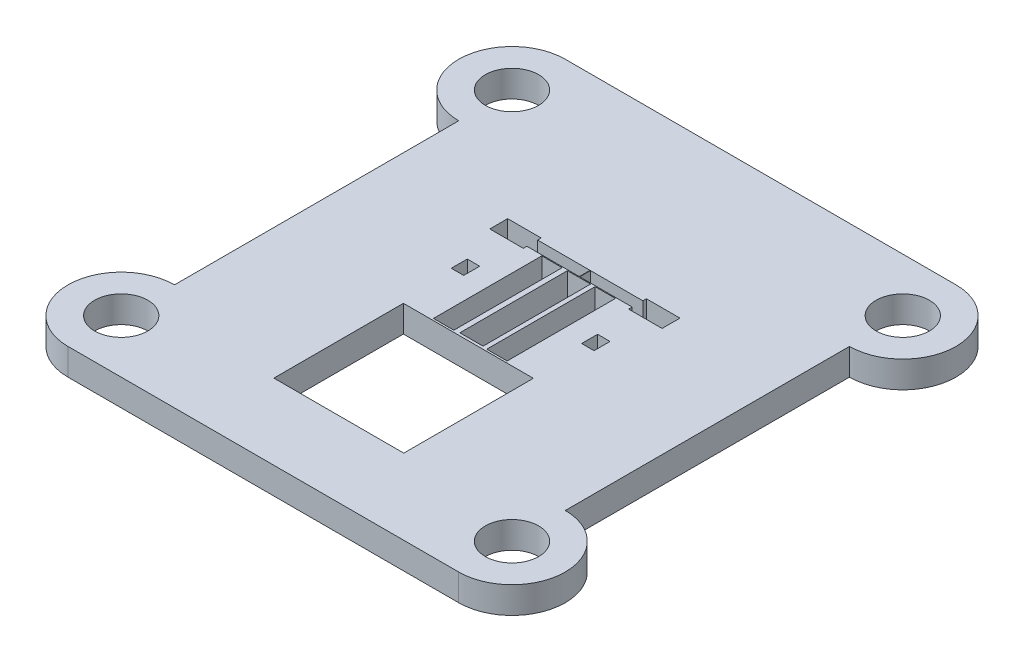
from build123d import *

# Parameters (mm, degrees)
SKETCH1_R           = 15
BOSS_EXTRUDE1_DEPTH = 15
CUT_EXTRUDE1_REACH  = 200.557
SKETCH6_W           = 73.144376366
SKETCH6_H           = 72.943161699
SKETCH6_W_2         = 11.5
SKETCH6_H_2         = 61
SKETCH6_W_3         = 13.06
SKETCH6_H_3         = 60.56
SKETCH6_W_4         = 7
SKETCH6_H_4         = 9
SKETCH7_W           = 22
SKETCH7_H           = 52
CUT_EXTRUDE2_DEPTH  = 10
FILLET1_R           = 1


with BuildPart() as part:
    # Sketch1 → Boss-Extrude1 (new body)
    with BuildSketch(Plane(origin=(0, 0, 0), x_dir=(1, 0, 0), z_dir=(0, 1, 0))):
        with BuildLine():
            Line((-110, -140), (80, -140))
            Line((80, -140), (80, 140))
            Line((80, 140), (-110, 140))
            ThreePointArc((-110, 140), (-140, 110), (-110, 80))
            Line((-110, 80), (-110, -80))
            ThreePointArc((-110, -80), (-140, -110), (-110, -140))
        make_face()
        with Locations(Location((-110, 110, 0), (0, 0, 270))):
            Circle(SKETCH1_R, mode=Mode.SUBTRACT)
        with Locations(Location((-110, -110, 0), (0, 0, 270))):
            Circle(SKETCH1_R, mode=Mode.SUBTRACT)
    boss_extrude1 = extrude(amount=BOSS_EXTRUDE1_DEPTH)

    # Mirror1: Boss-Extrude1 across plane
    add(boss_extrude1.mirror(Plane(origin=(0, 0, 0), x_dir=(0, 0, 1), z_dir=(1, 0, 0))))

    # Sketch6 → Cut-Extrude1 (cut, up to next)
    with BuildSketch(Plane(origin=(0, 15, 0), x_dir=(1, 0, 0), z_dir=(0, 1, 0)), mode=Mode.PRIVATE) as cut_extrude1_sk1:
        with Locations((0, -61.02841915)):
            Rectangle(SKETCH6_W, SKETCH6_H)
    cut_extrude1_tool1 = extrude(cut_extrude1_sk1.sketch, amount=-CUT_EXTRUDE1_REACH, mode=Mode.PRIVATE) & part.part
    # Sketch6 → Cut-Extrude1 (cut, up to next)
    with BuildSketch(Plane(origin=(0, 15, 0), x_dir=(1, 0, 0), z_dir=(0, 1, 0)), mode=Mode.PRIVATE) as cut_extrude1_sk2:
        with Locations((-15, 7)):
            Rectangle(SKETCH6_W_2, SKETCH6_H_2)
    cut_extrude1_tool2 = extrude(cut_extrude1_sk2.sketch, amount=-CUT_EXTRUDE1_REACH, mode=Mode.PRIVATE) & part.part
    # Sketch6 → Cut-Extrude1 (cut, up to next)
    with BuildSketch(Plane(origin=(0, 15, 0), x_dir=(1, 0, 0), z_dir=(0, 1, 0)), mode=Mode.PRIVATE) as cut_extrude1_sk3:
        Polygon((-0.14, 38), (-0.14, 44.06), (-29.63, 44.06), (-29.63, 46.06), (-48.5, 46.06), (-48.5, 36), (-29.63, 36), (-29.63, 38), align=None)
    cut_extrude1_tool3 = extrude(cut_extrude1_sk3.sketch, amount=-CUT_EXTRUDE1_REACH, mode=Mode.PRIVATE) & part.part
    # Sketch6 → Cut-Extrude1 (cut, up to next)
    with BuildSketch(Plane(origin=(0, 15, 0), x_dir=(1, 0, 0), z_dir=(0, 1, 0)), mode=Mode.PRIVATE) as cut_extrude1_sk4:
        Polygon((29.63, 36), (48.5, 36), (48.5, 46.06), (29.63, 46.06), (29.63, 44.06), (0.14, 44.06), (0.14, 38), (29.63, 38), align=None)
    cut_extrude1_tool4 = extrude(cut_extrude1_sk4.sketch, amount=-CUT_EXTRUDE1_REACH, mode=Mode.PRIVATE) & part.part
    # Sketch6 → Cut-Extrude1 (cut, up to next)
    with BuildSketch(Plane(origin=(0, 15, 0), x_dir=(1, 0, 0), z_dir=(0, 1, 0)), mode=Mode.PRIVATE) as cut_extrude1_sk5:
        with Locations((0.22, 7.22)):
            Rectangle(SKETCH6_W_3, SKETCH6_H_3)
    cut_extrude1_tool5 = extrude(cut_extrude1_sk5.sketch, amount=-CUT_EXTRUDE1_REACH, mode=Mode.PRIVATE) & part.part
    # Sketch6 → Cut-Extrude1 (cut, up to next)
    with BuildSketch(Plane(origin=(0, 15, 0), x_dir=(1, 0, 0), z_dir=(0, 1, 0)), mode=Mode.PRIVATE) as cut_extrude1_sk6:
        with Locations((15, 7)):
            Rectangle(SKETCH6_W_2, SKETCH6_H_2)
    cut_extrude1_tool6 = extrude(cut_extrude1_sk6.sketch, amount=-CUT_EXTRUDE1_REACH, mode=Mode.PRIVATE) & part.part
    # Sketch6 → Cut-Extrude1 (cut, up to next)
    with BuildSketch(Plane(origin=(0, 15, 0), x_dir=(1, 0, 0), z_dir=(0, 1, 0)), mode=Mode.PRIVATE) as cut_extrude1_sk7:
        with Locations((-36.69, 10.5)):
            Rectangle(SKETCH6_W_4, SKETCH6_H_4)
    cut_extrude1_tool7 = extrude(cut_extrude1_sk7.sketch, amount=-CUT_EXTRUDE1_REACH, mode=Mode.PRIVATE) & part.part
    # Sketch6 → Cut-Extrude1 (cut, up to next)
    with BuildSketch(Plane(origin=(0, 15, 0), x_dir=(1, 0, 0), z_dir=(0, 1, 0)), mode=Mode.PRIVATE) as cut_extrude1_sk8:
        with Locations((36.69, 10.5)):
            Rectangle(SKETCH6_W_4, SKETCH6_H_4)
    cut_extrude1_tool8 = extrude(cut_extrude1_sk8.sketch, amount=-CUT_EXTRUDE1_REACH, mode=Mode.PRIVATE) & part.part
    add(cut_extrude1_tool1.solids().sort_by_distance((0, 15, 61.028419))[0], mode=Mode.SUBTRACT)
    add(cut_extrude1_tool2.solids().sort_by_distance((-15, 15, -7))[0], mode=Mode.SUBTRACT)
    add(cut_extrude1_tool3.solids().sort_by_distance((-27.339883, 15, -41.03))[0], mode=Mode.SUBTRACT)
    add(cut_extrude1_tool4.solids().sort_by_distance((27.339883, 15, -41.03))[0], mode=Mode.SUBTRACT)
    add(cut_extrude1_tool5.solids().sort_by_distance((0.22, 15, -7.22))[0], mode=Mode.SUBTRACT)
    add(cut_extrude1_tool6.solids().sort_by_distance((15, 15, -7))[0], mode=Mode.SUBTRACT)
    add(cut_extrude1_tool7.solids().sort_by_distance((-36.69, 15, -10.5))[0], mode=Mode.SUBTRACT)
    add(cut_extrude1_tool8.solids().sort_by_distance((36.69, 15, -10.5))[0], mode=Mode.SUBTRACT)

    # Sketch7 → Cut-Extrude2 (cut)
    with BuildSketch(Plane.XZ):
        with Locations((49, -88.06497659)):
            Rectangle(SKETCH7_W, SKETCH7_H)
        with Locations((-49, -88.06497659)):
            Rectangle(SKETCH7_W, SKETCH7_H)
    extrude(amount=-CUT_EXTRUDE2_DEPTH, mode=Mode.SUBTRACT)

    # Fillet1
    fillet1_edges = [part.edges().sort_by_distance(p)[0] for p in [
        (60, 10, -88.06497659),
        (49, 10, -114.06497659),
        (38, 10, -88.06497659),
        (49, 10, -62.06497659),
        (60, 0, -88.06497659),
        (49, 0, -62.06497659),
        (38, 0, -88.06497659),
        (49, 0, -114.06497659),
        (-60, 10, -88.06497659),
        (-49, 10, -62.06497659),
        (-38, 10, -88.06497659),
        (-49, 10, -114.06497659),
        (-60, 0, -88.06497659),
        (-49, 0, -114.06497659),
        (-38, 0, -88.06497659),
        (-49, 0, -62.06497659),
    ]]
    fillet(fillet1_edges, radius=FILLET1_R)


solid = part.part
